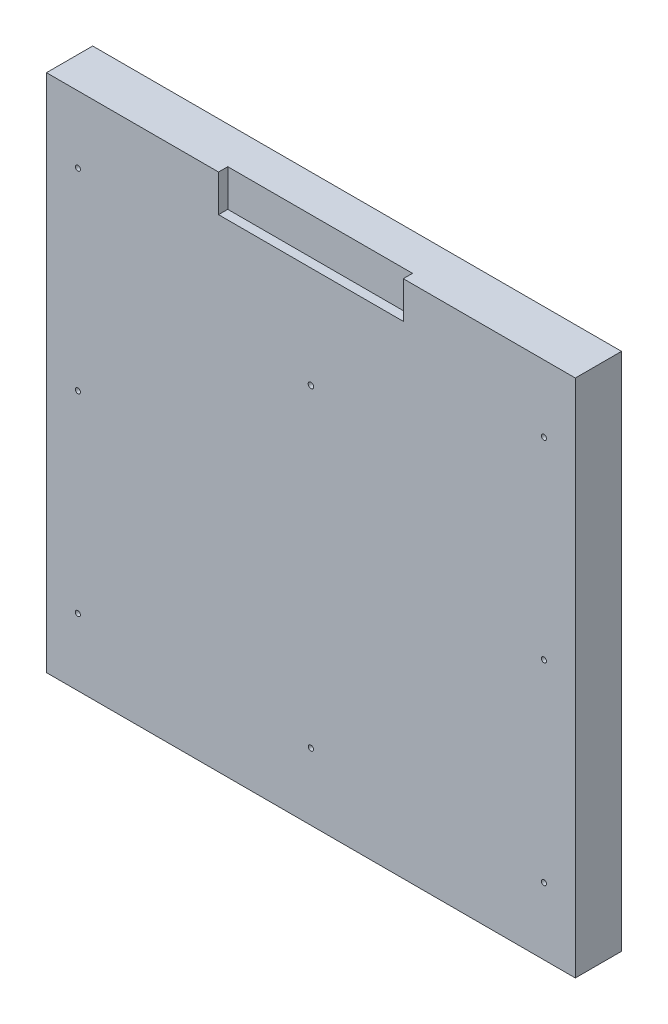
from build123d import *

# Parameters (mm, degrees)
SKETCH_1_W               = 1145
SKETCH_1_H               = 1125
EXTRUDE_1_DEPTH          = 100
SKETCH_2_W               = 400
SKETCH_2_H               = 160
CUT_EXTRUDE_1_DEPTH      = 20
CUT_EXTRUDE_2_DEPTH      = 809.803128085
CUT_EXTRUDE_2_DEPTH_BACK = 809.803128085
SKETCH_4_R               = 5.5
CUT_EXTRUDE_3_DEPTH      = 809.803128085
CUT_EXTRUDE_3_DEPTH_BACK = 809.803128085
SKETCH_3_R               = 6


with BuildPart() as part:
    # 草图1 → 凸台-拉伸1 (new body)
    with BuildSketch(Plane.XY):
        Rectangle(SKETCH_1_W, SKETCH_1_H)
    extrude(amount=EXTRUDE_1_DEPTH)

    # 草图2 → 切除-拉伸1 (cut)
    with BuildSketch(Plane.XY.offset(100)):
        with Locations((0, 562.5)):
            Rectangle(SKETCH_2_W, SKETCH_2_H)
    extrude(amount=-CUT_EXTRUDE_1_DEPTH, mode=Mode.SUBTRACT)

    # 草图4 → 切除-拉伸2 (cut, two sides: drawn at the far end of the back side and taken through both)
    with BuildSketch(Plane.XY.offset(100).offset(-CUT_EXTRUDE_2_DEPTH_BACK)):
        with Locations((-504.5, 417.5)):
            Circle(SKETCH_4_R)
        with Locations((-504.5, -417.5)):
            Circle(SKETCH_4_R)
        with Locations((504.5, -417.5)):
            Circle(SKETCH_4_R)
        with Locations((504.5, 417.5)):
            Circle(SKETCH_4_R)
        with Locations((0, -417.5)):
            Circle(SKETCH_4_R)
        with Locations((-504.5, 0)):
            Circle(SKETCH_4_R)
        with Locations((504.5, 0)):
            Circle(SKETCH_4_R)
    extrude(amount=CUT_EXTRUDE_2_DEPTH + CUT_EXTRUDE_2_DEPTH_BACK, mode=Mode.SUBTRACT)

    # 草图3 → 切除-拉伸3 (cut, two sides: drawn at the far end of the back side and taken through both)
    with BuildSketch(Plane.XY.offset(100).offset(-CUT_EXTRUDE_3_DEPTH_BACK)):
        with Locations((0, 262.5)):
            Circle(SKETCH_3_R)
    extrude(amount=CUT_EXTRUDE_3_DEPTH + CUT_EXTRUDE_3_DEPTH_BACK, mode=Mode.SUBTRACT)


solid = part.part
